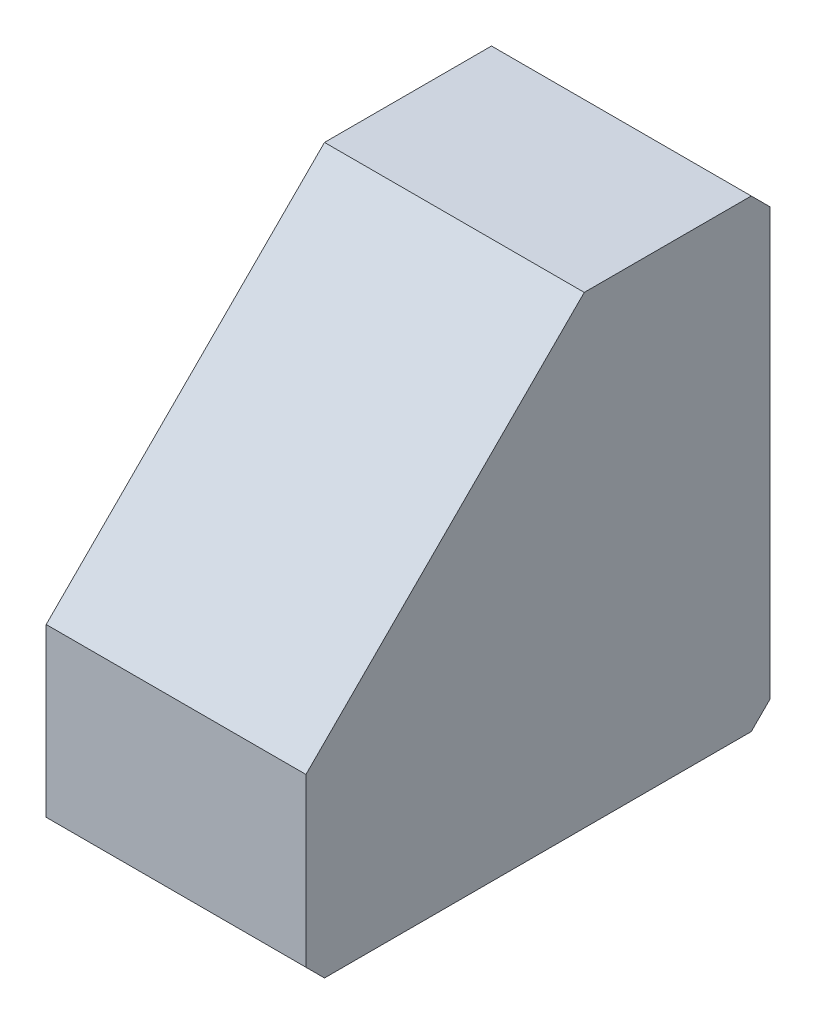
SolidWorks part; units mm, degrees
material "AL6061"
ref_plane "Front Plane" through (0, 0, 0) normal (0, 0, 1) x (1, 0, 0)
ref_plane "Top Plane" through (0, 0, 0) normal (0, 1, 0) x (1, 0, 0)
ref_plane "Right Plane" through (0, 0, 0) normal (1, 0, 0) x (0, 0, -1)
sketch "Sketch1" plane through (0, 0, 0) normal (1, 0, 0) x (0, 0, -1)
  line L0 (0, 0) -> (0, 25)
  line L1 (0, 25) -> (-10, 25)
  line L2 (-10, 25) -> (-25, 10)
  line L3 (-25, 10) -> (-25, 0)
  line L4 (-25, 0) -> (0, 0)
  dimension "D1" = 10
  dimension "D2" = 10
  dimension "D3" = 25
  dimension "D4" = 25
extrude "Boss-Extrude1" add sketch "Sketch1" along normal mid plane 14
hole_wizard "M6 Tapped Hole1" positions "Sketch2" profile "Sketch3" tap size "M6" standard "GB"
sketch "Sketch2" plane through (0, 0, 0) normal (0, -1, 0) x (-1, 0, 0)
  line L0 (0, 0) -> (0, -30.1036) construction
  line L1 (-7, 0) -> (7, 0) construction
  point P7 (0, -15)
  dimension "D1" = 15
sketch "Sketch3" plane through (0, 0, 15) normal (1, 0, 0) x (0, 0, -1)
  line L0 (0, 0) -> (0, 16.5022)
  line L1 (0, 16.5022) -> (2.5, 15)
  line L2 (2.5, 15) -> (2.5, 0)
  line L5 (2.5, 0) -> (0, 0)
  line L10 (0, 16.5022) -> (-2.5, 15) construction
  line L11 (0, -6.35) -> (0, 107.95) construction
  dimension "螺纹孔钻头直径" = 5
  dimension "螺纹孔钻头深度" = 15
  dimension "导头角度" = 118
cosmetic thread "Cosmetic Thread1" parameters "D1"=12, "D2"=6
hole_wizard "M6 Tapped Hole2" positions "Sketch4" profile "Sketch5" tap size "M6" standard "GB"
sketch "Sketch4" plane through (0, 0, 0) normal (0, 0, -1) x (-1, 0, 0)
  line L0 (0, 0) -> (0, 58.1081) construction
  line L1 (-7, 0) -> (7, 0) construction
  point P7 (0, 15)
  dimension "D1" = 15
sketch "Sketch5" plane through (0, 15, 0) normal (1, 0, 0) x (0, 1, 0)
  line L0 (0, 0) -> (0, 16.5022)
  line L1 (0, 16.5022) -> (2.5, 15)
  line L2 (2.5, 15) -> (2.5, 0)
  line L5 (2.5, 0) -> (0, 0)
  line L10 (0, 16.5022) -> (-2.5, 15) construction
  line L11 (0, -6.35) -> (0, 107.95) construction
  dimension "螺纹孔钻头直径" = 5
  dimension "螺纹孔钻头深度" = 15
  dimension "导头角度" = 118
cosmetic thread "Cosmetic Thread3" parameters "D1"=12, "D2"=6
chamfer "Chamfer1" distance 1 angle 45 3 edges at (0, 0, 25) (0, 25, 0) (0, 0, 0)
